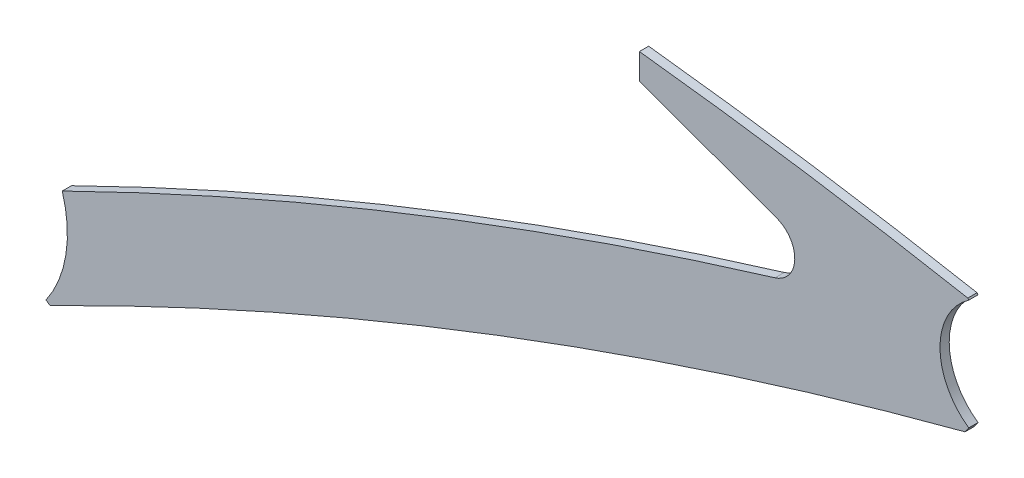
SolidWorks part; units mm, degrees
ref_plane "Front Plane" through (0, 0, 0) normal (0, 0, 1) x (1, 0, 0)
ref_plane "Top Plane" through (0, 0, 0) normal (0, 1, 0) x (1, 0, 0)
ref_plane "Right Plane" through (0, 0, 0) normal (1, 0, 0) x (0, 0, -1)
sketch "Sketch1" plane through (0, 0, 0) normal (0, 0, 1) x (1, 0, 0)
  line L0 (1144.5, 470.0019) -> (1144.5, 190.0307) construction
  line L1 (1102.6289, 305.7019) -> (1098.6321, 299.9938)
  line L2 (1144.5, 365.5) -> (1170.2562, 365.5) construction
  line L3 (1144.5, 365.5) -> (849.4851, 365.5) construction
  line L4 (1102.6289, 425.2981) -> (1101.5994, 426.7684)
  line L5 (104.8515, -73.4178) -> (109.2346, -76.4869)
  line L6 (0, 0) -> (335.2665, 0) construction
  line L7 (1069.0035, 426.3) -> (1267.1437, 426.3) construction
  line L8 (1094.2396, 302.4) -> (1107.7932, 302.4) construction
  line L9 (746.5, 480.1) -> (746.5, 452.4)
  line L10 (-47.1258, -82.1) -> (319.2225, -82.1) construction
  line L11 (746.5, 480.1) -> (746.5, 244.0599) construction
  line L12 (746.5, 452.4) -> (894.7706, 398.4339)
  line L15 (842.5, 371.3917) -> (842.5, 244.0599) construction
  line L16 (943.6773, 356.5627) -> (943.6773, 356.5627) construction
  line L17 (943.6773, 356.5627) -> (943.6773, 356.5627) construction
  line L18 (209.5245, 79.2181) -> (209.5245, 79.2181) construction
  arc A0 (104.8515, -73.4178) -> (122.4139, 37.4011) centre (0, 0) ccw
  arc A1 (1102.6289, 425.2981) -> (1102.6289, 305.7019) centre (1144.5, 365.5) ccw
  arc A2 (1101.5994, 426.7684) -> (746.5, 480.1) centre (184.2965, -4472.0897) ccw
  arc A3 (1098.6321, 299.9938) -> (109.2346, -76.4869) centre (2376.4255, -4546.385) ccw
  arc A4 (943.6773, 356.5627) -> (209.5245, 79.2181) centre (2376.4255, -4546.385) ccw construction
  arc A5 (893.2211, 341.5357) -> (894.7706, 398.4339) centre (884.51, 370.2431) ccw
  arc A6 (893.2211, 341.5357) -> (122.4139, 37.4011) centre (2376.4255, -4546.385) ccw
  arc A7 (104.8515, -73.4178) -> (98.2018, -82.1) centre (0, 0) ccw construction
  arc A8 (209.5245, 79.2181) -> (171.8531, -143.675) centre (0, 0) ccw construction
  arc A9 (943.6773, 356.5627) -> (842.5, 371.3917) centre (184.2965, -4472.0897) ccw construction
  arc A10 (943.6773, 356.5627) -> (943.6773, 356.5627) centre (943.6773, 356.5627) cw construction
  point P21 (1104.0975, 426.3)
  point P26 (1107.7932, 302.4)
  point P27 (98.2018, -82.1)
  dimension "D1" = 256
  dimension "D4" = 146
  dimension "D5" = 35
  dimension "D12" = 9968
  dimension "D14" = 10024
  dimension "D18" = 30
  dimension "D2" = 365.5
  dimension "D3" = 1144.5
  dimension "D7" = 55
  dimension "D8" = 55
  dimension "D6" = 60.8
  dimension "D9" = 63.1
  dimension "D10" = 398
  dimension "D11" = 114.6
  dimension "D13" = 82.1
  dimension "D16" = 86.9
  dimension "D17" = 20
  dimension "D15" = 96
extrude "Boss-Extrude1" add sketch "Sketch1" along normal blind 10 contours A5 A6 A0 L5 A3 L1 A1 L4 A2 L9 L12
